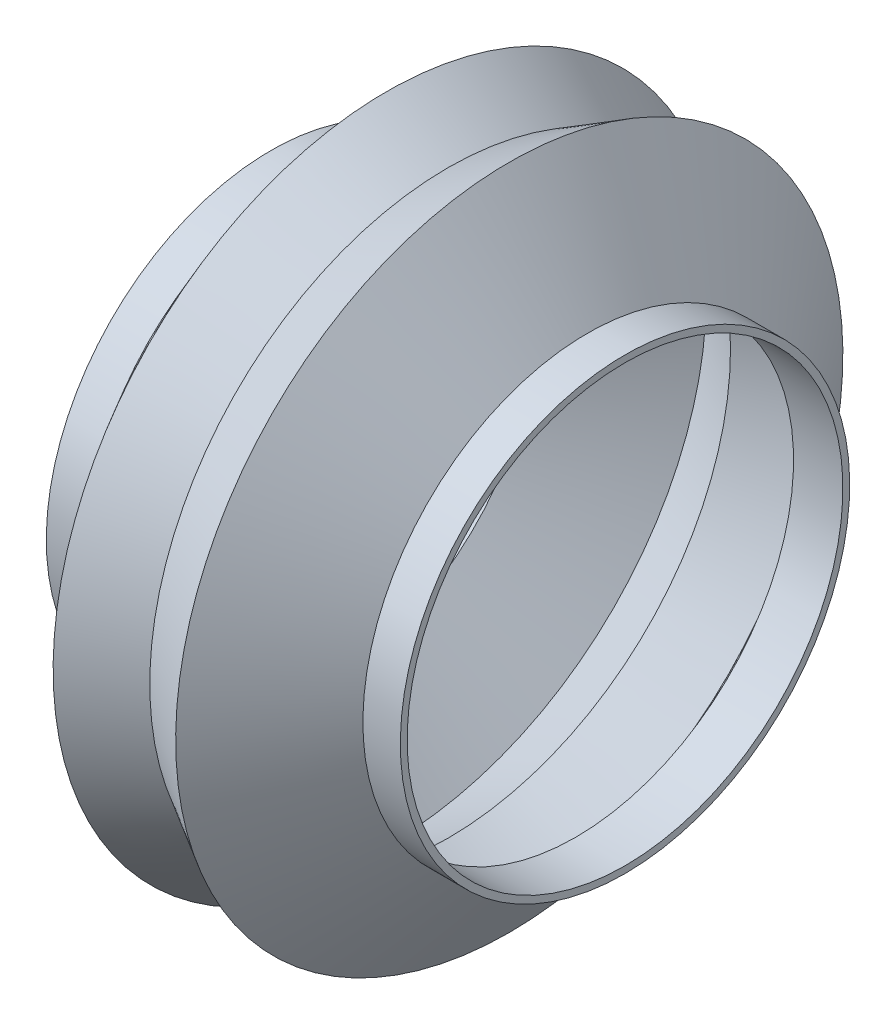
from build123d import *

# Parameters (mm, degrees)
SKETCH4_R          = 16
CUT_EXTRUDE2_DEPTH = 120


with BuildPart() as part:
    # Sketch1 → Revolve1 (revolve)
    with BuildSketch(Plane.XY, mode=Mode.PRIVATE) as revolve1_sk:
        Polygon((0, 21.901923789), (4.5, 24.5), (10.25, 16.5), (13, 16.5), (13, 0), (-13, 0), (-13, 16.5), (-10.25, 16.5), (-4.5, 24.5), align=None)
    revolve(revolve1_sk.sketch.rotate(Axis((-38.0976844, 0, 0), (1, 0, 0)), 180), axis=Axis((-38.0976844, 0, 0), (1, 0, 0)))

    # Sketch3 → Cut-Revolve1 (revolve, cut)
    with BuildSketch(Plane.XY):
        Polygon((4.216204142, 23.181449847), (0, 20.74722325), (-4.216204142, 23.181449847), (-9.737246219, 15.5), (-12, 15.5), (-12, 1), (-12, 0), (12, 0), (12, 1), (12, 15.5), (9.737246219, 15.5), align=None)
    revolve(axis=Axis((12, 0, 0), (-1, 0, 0)), mode=Mode.SUBTRACT)

    # Sketch4 → Cut-Extrude2 (cut)
    with BuildSketch(Plane(origin=(13, 0, 0), x_dir=(0, 0, -1), z_dir=(1, 0, 0))):
        with Locations(Location((0, 0, 0), (0, 0, 90))):
            Circle(SKETCH4_R)
    extrude(amount=-CUT_EXTRUDE2_DEPTH, mode=Mode.SUBTRACT)


solid = part.part
